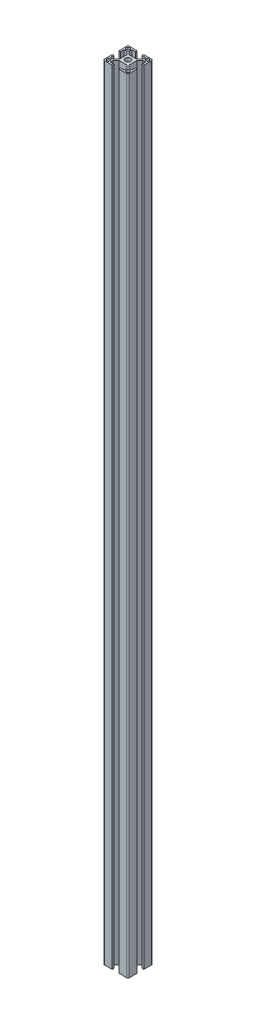
SolidWorks part; units mm, degrees
ref_plane "前视基准面" through (0, 0, 0) normal (0, 0, 1) x (1, 0, 0)
ref_plane "上视基准面" through (0, 0, 0) normal (0, 1, 0) x (1, 0, 0)
ref_plane "右视基准面" through (0, 0, 0) normal (1, 0, 0) x (0, 0, -1)
sketch "草图1" plane through (0, 0, 0) normal (0, 1, 0) x (1, 0, 0)
  line L44 (6.75, -28) -> (11, -28)
  line L45 (11, -28) -> (11, -30)
  line L46 (11, -30) -> (2, -30)
  line L47 (0, -28) -> (0, -19)
  line L48 (0, -19) -> (2, -19)
  line L49 (2, -19) -> (2, -23.25)
  line L50 (28, -30) -> (19, -30)
  line L51 (19, -30) -> (19, -28)
  line L52 (23.25, -28) -> (23.25, -24.6642)
  line L53 (19, -28) -> (23.25, -28)
  line L54 (30, -19) -> (30, -28)
  line L55 (28, -19) -> (30, -19)
  line L56 (28, -23.25) -> (28, -19)
  line L57 (24.6642, -23.25) -> (28, -23.25)
  line L58 (21, -19.5858) -> (24.6642, -23.25)
  line L59 (23.25, -24.6642) -> (19.5858, -21)
  line L60 (6.75, -24.6642) -> (6.75, -28)
  line L61 (2, -23.25) -> (5.3358, -23.25)
  line L62 (5.3358, -23.25) -> (9, -19.5858)
  line L63 (10.4142, -21) -> (6.75, -24.6642)
  line L64 (19.5858, -21) -> (10.4142, -21)
  line L65 (9, -19.5858) -> (9, -10.4142)
  line L66 (21, -10.4142) -> (21, -19.5858)
  line L67 (30, -11) -> (28, -11)
  line L68 (28, -11) -> (28, -6.75)
  line L69 (28, -6.75) -> (24.6642, -6.75)
  line L70 (24.6642, -6.75) -> (21, -10.4142)
  line L71 (19.5858, -9) -> (23.25, -5.3358)
  line L72 (10.4142, -9) -> (19.5858, -9)
  line L73 (6.75, -5.3358) -> (10.4142, -9)
  line L74 (9, -10.4142) -> (5.3358, -6.75)
  line L75 (2, -11) -> (0, -11)
  line L76 (2, -6.75) -> (2, -11)
  line L77 (5.3358, -6.75) -> (2, -6.75)
  line L78 (6.75, -2) -> (6.75, -5.3358)
  line L79 (23.25, -5.3358) -> (23.25, -2)
  line L80 (23.25, -2) -> (19, -2)
  line L81 (19, -2) -> (19, 0)
  line L82 (11, 0) -> (11, -2)
  line L83 (11, -2) -> (6.75, -2)
  line L84 (30, -2) -> (30, -11)
  line L85 (19, 0) -> (28, 0)
  line L86 (2, 0) -> (11, 0)
  line L87 (0, -11) -> (0, -2)
  line L88 (0, -15) -> (30, -15) construction
  line L89 (15, -30) -> (15, 0) construction
  line L90 (0, 0) -> (30, -30) construction
  line L91 (0, -30) -> (30, 0) construction
  arc A9 (0, -28) -> (2, -30) centre (2, -28) ccw
  circle A10 centre (3.375, -26.625) radius 2.1
  circle A11 centre (26.625, -26.625) radius 2.1
  arc A12 (28, -30) -> (30, -28) centre (28, -28) ccw
  circle A13 centre (15, -15) radius 3.4
  circle A14 centre (3.375, -3.375) radius 2.1
  circle A15 centre (26.625, -3.375) radius 2.1
  arc A16 (30, -2) -> (28, 0) centre (28, -2) ccw
  arc A17 (2, 0) -> (0, -2) centre (2, -2) ccw
  dimension "D2" = 15
  dimension "D5" = 6.8
  dimension "D8" = 6
  dimension "D11" = 23.25
  dimension "D12" = 3.375
  dimension "D13" = 23.25
  dimension "D14" = 4.2
  dimension "D15" = 2
  dimension "D16" = 2
  dimension "D23" = 2
  dimension "D24" = 2
  dimension "D1" = 15
  dimension "D3" = 45
  dimension "D4" = 45
  dimension "D6" = 30
  dimension "D7" = 30
  dimension "D9" = 12
  dimension "D10" = 3.375
  dimension "D17" = 11
  dimension "D18" = 8
  dimension "D19" = 2
  dimension "D20" = 2
  dimension "D21" = 11
  dimension "D22" = 8
  dimension "D25" = 2
  dimension "D26" = 2
  dimension "D27" = 6.75
  dimension "D28" = 16.5
  dimension "D29" = 6.75
  dimension "D30" = 16.5
  dimension "D31" = 12
  dimension "D32" = 6
  dimension "D33" = 2
  dimension "D34" = 1
  dimension "D35" = 2
  dimension "D36" = 1
extrude "拉伸1" add sketch "草图1" along normal blind 940
hole_wizard "打孔尺寸根据内六角圆柱头螺钉的类型1" positions "草图3" profile "草图2" counterbore size "M6" standard "GB" end condition through all
sketch "草图3" plane through (0, 0, 0) normal (0, 0, -1) x (-1, 0, 0)
  line L1 (-15, 940) -> (-15, 0) construction
  line L2 (-19.5858, 940) -> (-10.4142, 940) construction
  line L3 (-19.5858, 0) -> (-10.4142, 0) construction
  line L6 (-11, 940) -> (-2, 940) construction
  line L8 (-11, 0) -> (-2, 0) construction
  point P0 (-15, 895)
  point P1 (-15, 545)
  point P3 (-15, 45)
  point P33 (-15, 395)
  dimension "D1" = 45
  dimension "D2" = 350
  dimension "D3" = 45
  dimension "D4" = 350
sketch "草图2" plane through (15, 895, 0) normal (1, 0, 0) x (0, 1, 0)
  line L0 (0, 0) -> (0, 30)
  line L1 (0, 30) -> (3.3, 30)
  line L3 (3.3, 30) -> (3.3, 9)
  line L4 (3.3, 9) -> (5.5, 9)
  line L5 (5.5, 9) -> (5.5, 0)
  line L7 (5.5, 0) -> (0, 0)
  line L11 (0, -6.35) -> (0, 107.95) construction
  dimension "通孔孔直径" = 6.6
  dimension "通孔孔深度" = 30
  dimension "柱形沉头孔直径" = 11
  dimension "柱形沉头孔深度" = 9
